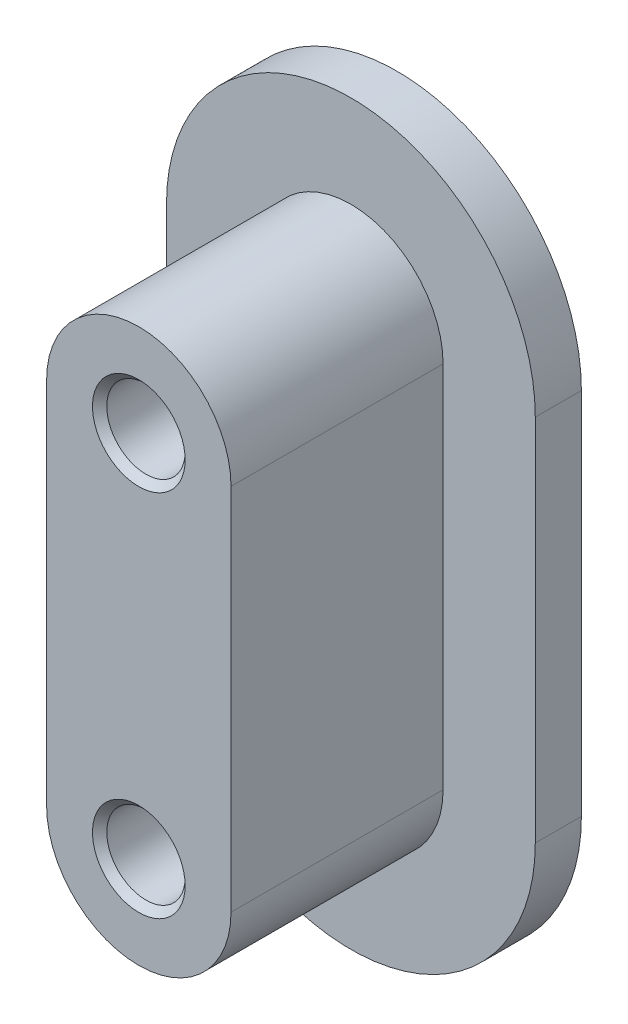
from build123d import *

# Parameters (mm, degrees)
EXTRUDE_1_DEPTH               = 28
EXTRUDE_2_DEPTH               = 5
HOLE_WIZARD_M10_1_D           = 8.5
HOLE_WIZARD_M10_1_DEPTH       = 21.946342369
HOLE_WIZARD_M10_1_CSINK_D     = 10.05
HOLE_WIZARD_M10_1_CSINK_ANGLE = 90
HOLE_WIZARD_M10_1_TIP         = 2.553657631


with BuildPart() as part:
    # 草图1 → 凸台-拉伸1 (new body)
    with BuildSketch(Plane.XY):
        with BuildLine():
            Line((-60, -60), (-60, -100))
            ThreePointArc((-60, -100), (-70, -110), (-80, -100))
            Line((-80, -100), (-80, -60))
            ThreePointArc((-80, -60), (-70, -50), (-60, -60))
        make_face()
    extrude(amount=EXTRUDE_1_DEPTH)

    # 草图2 → 凸台-拉伸2 (add)
    with BuildSketch(Plane.XY):
        with BuildLine():
            Line((-90, -60), (-90, -100))
            ThreePointArc((-90, -100), (-70, -120), (-50, -100))
            Line((-50, -100), (-50, -60))
            ThreePointArc((-50, -60), (-70, -40), (-90, -60))
        make_face()
    extrude(amount=EXTRUDE_2_DEPTH)

    # M10 螺纹孔1
    with Locations(Plane.XY.offset(28)):
        with Locations((-70, -60), (-70, -100)):
            CounterSinkHole(HOLE_WIZARD_M10_1_D / 2, HOLE_WIZARD_M10_1_CSINK_D / 2, depth=HOLE_WIZARD_M10_1_DEPTH, counter_sink_angle=HOLE_WIZARD_M10_1_CSINK_ANGLE)
            with Locations((0, 0, -(HOLE_WIZARD_M10_1_DEPTH + HOLE_WIZARD_M10_1_TIP / 2))):  # 118° drill point
                Cone(0, HOLE_WIZARD_M10_1_D / 2, HOLE_WIZARD_M10_1_TIP, mode=Mode.SUBTRACT)


solid = part.part
